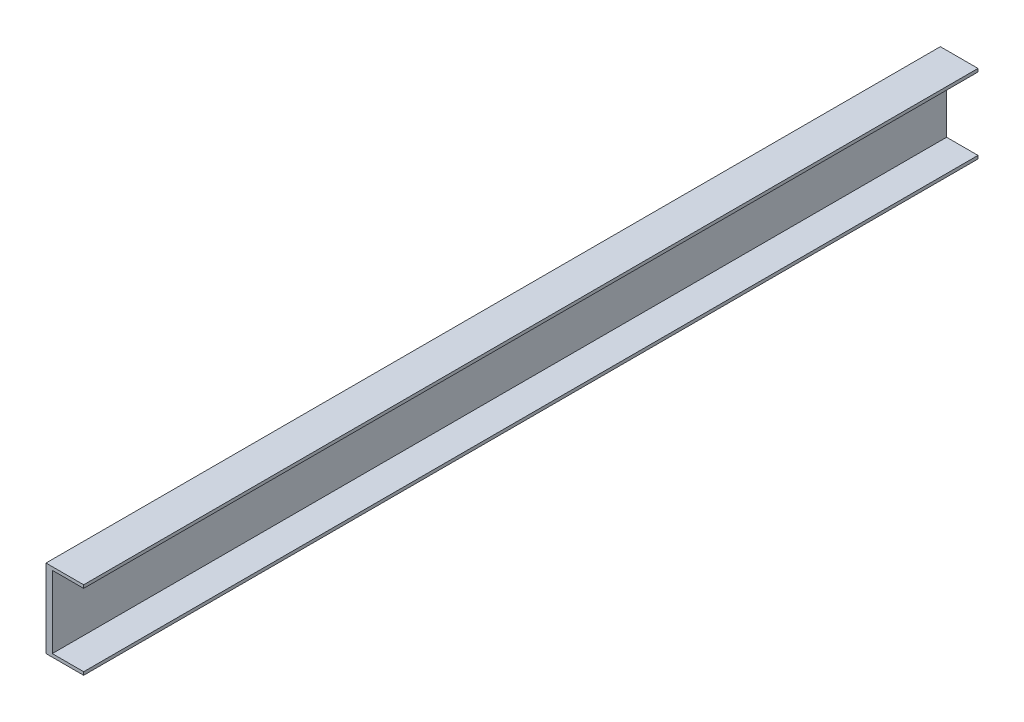
from build123d import *

# Parameters (mm, degrees)
EXTRUDE1_DEPTH = 1140


with BuildPart() as part:
    # Sketch1 → Extrude1 (new body)
    with BuildSketch(Plane.XY):
        Polygon((0, 0), (-48, 0), (-48, 100), (0, 100), (0, 96), (-40, 96), (-40, 4), (0, 4), align=None)
    extrude(amount=EXTRUDE1_DEPTH)


solid = part.part
